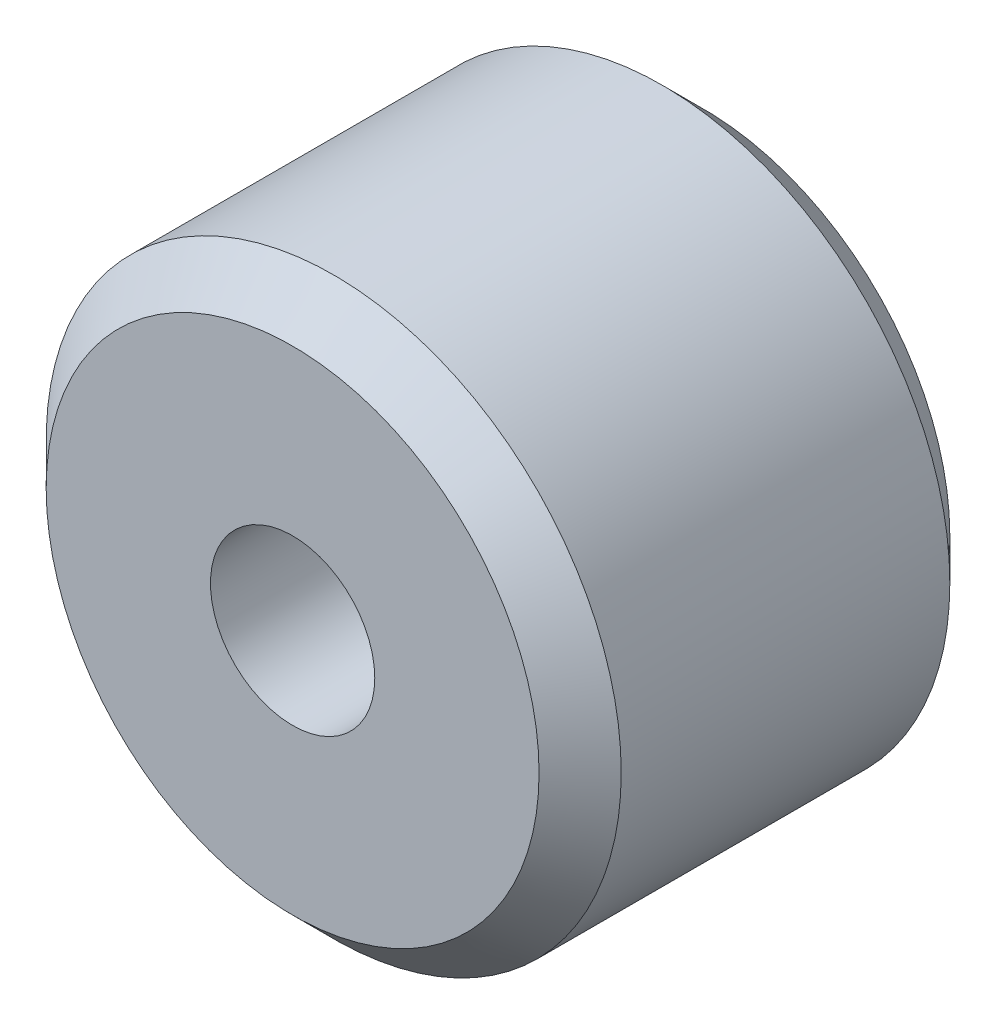
from build123d import *

# Parameters (mm, degrees)
SKETCH1_R           = 3.5
BOSS_EXTRUDE1_DEPTH = 5
SKETCH2_R           = 1
CUT_EXTRUDE1_DEPTH  = 11
CHAMFER1_SIZE       = 0.5


with BuildPart() as part:
    # Sketch1 → Boss-Extrude1 (new body)
    with BuildSketch(Plane.XY):
        Circle(SKETCH1_R)
    extrude(amount=BOSS_EXTRUDE1_DEPTH)

    # Sketch2 → Cut-Extrude1 (cut)
    with BuildSketch(Plane.XY.offset(5)):
        Circle(SKETCH2_R)
    extrude(amount=-CUT_EXTRUDE1_DEPTH, mode=Mode.SUBTRACT)

    # Chamfer1
    chamfer1_edges = [part.edges().sort_by_distance(p)[0] for p in [
        (-3.5, 0, 0),
        (-3.5, 0, 5),
    ]]
    chamfer(chamfer1_edges, length=CHAMFER1_SIZE)


solid = part.part
